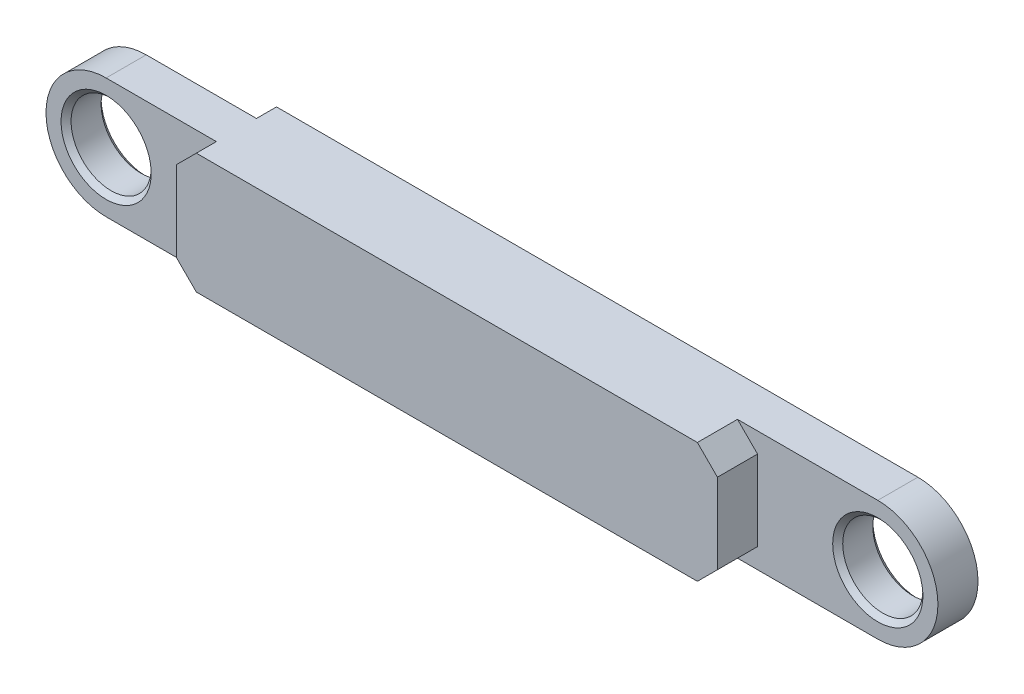
from build123d import *

# Parameters (mm, degrees)
BOSS_EXTRUDE1_DEPTH = 4
SKETCH2_R           = 4
CUT_EXTRUDE2_DEPTH  = 45.634627813
SKETCH3_W           = 18
SKETCH3_H           = 4
SKETCH3_W_2         = 15
SKETCH3_H_2         = 2
CUT_EXTRUDE3_DEPTH  = 46.30176597
CHAMFER1_SIZE       = 2
CHAMFER2_SIZE       = 0.5


with BuildPart() as part:
    # Sketch1 → Boss-Extrude1 (new, symmetric)
    with BuildSketch(Plane.XY):
        with BuildLine():
            Line((-37.5, 6), (37.5, 6))
            ThreePointArc((37.5, 6), (43.5, 0), (37.5, -6))
            Line((37.5, -6), (-37.5, -6))
            ThreePointArc((-37.5, -6), (-43.5, 0), (-37.5, 6))
        make_face()
    extrude(amount=BOSS_EXTRUDE1_DEPTH, both=True)

    # Sketch2 → Cut-Extrude2 (cut, through all)
    with BuildSketch(Plane.XY.offset(4)):
        with Locations((37.5, 0)):
            Circle(SKETCH2_R)
        with Locations((-37.5, 0)):
            Circle(SKETCH2_R)
    extrude(amount=-CUT_EXTRUDE2_DEPTH, mode=Mode.SUBTRACT)

    # Sketch3 → Cut-Extrude3 (cut, through all)
    with BuildSketch(Plane(origin=(0, 6, 0), x_dir=(1, 0, 0), z_dir=(0, 1, 0))):
        with Locations((34.5, -2)):
            Rectangle(SKETCH3_W, SKETCH3_H)
        with Locations((-36, -3)):
            Rectangle(SKETCH3_W_2, SKETCH3_H_2)
        with Locations((-36, 3)):
            Rectangle(SKETCH3_W_2, SKETCH3_H_2)
    extrude(amount=-CUT_EXTRUDE3_DEPTH, mode=Mode.SUBTRACT)

    # Chamfer1
    chamfer1_edges = [part.edges().sort_by_distance(p)[0] for p in [
        (25.5, -6, 2),
        (25.5, 6, 2),
        (-28.5, 6, 3),
        (-28.5, -6, 3),
        (-28.5, -6, -3),
        (-28.5, 6, -3),
    ]]
    chamfer(chamfer1_edges, length=CHAMFER1_SIZE)

    # Chamfer2
    chamfer2_edges = [part.edges().sort_by_distance(p)[0] for p in [
        (33.5, 0, -4),
        (33.5, 0, 0),
        (-41.5, 0, 2),
        (-41.5, 0, -2),
    ]]
    chamfer(chamfer2_edges, length=CHAMFER2_SIZE)


solid = part.part
